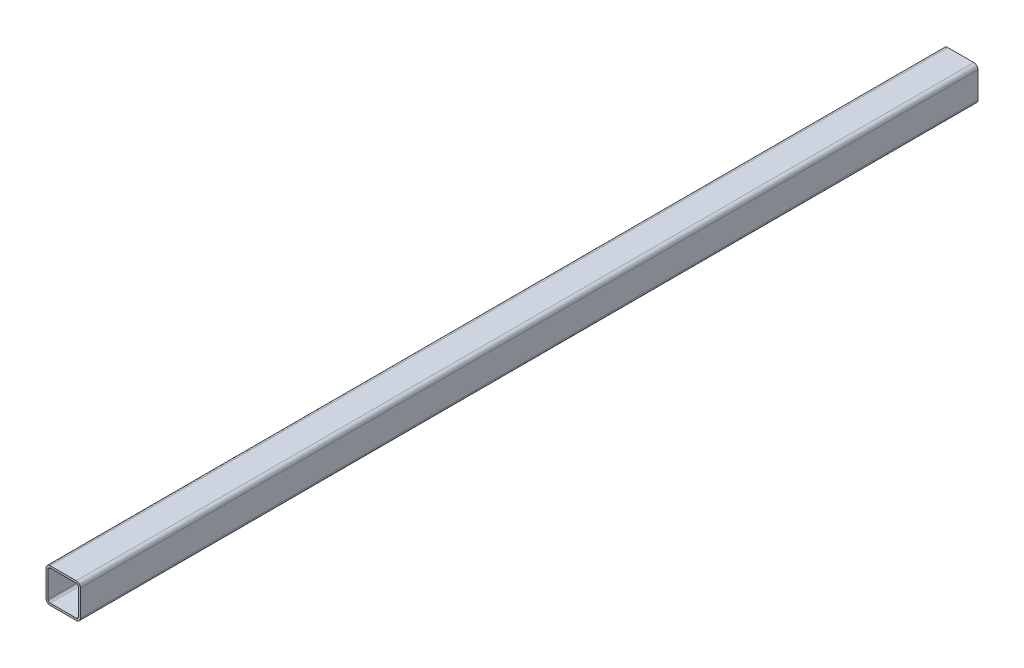
from build123d import *

# Parameters (mm, degrees)
GB_6728_1986_050_X_50_X_3_1_DEPTH = 1305


with BuildPart() as part:
    # Sketch1 → Gb／6728-1986方形空心型钢 050 X 50 X 3(1) (new body)
    with BuildSketch(Plane.YX.offset(-652.5)):
        with BuildLine():
            Line((-19, -25), (19, -25))
            ThreePointArc((19, -25), (23.242640687, -23.242640687), (25, -19))
            Line((25, -19), (25, 19))
            ThreePointArc((25, 19), (23.242640687, 23.242640687), (19, 25))
            Line((19, 25), (-19, 25))
            ThreePointArc((-19, 25), (-23.242640687, 23.242640687), (-25, 19))
            Line((-25, 19), (-25, -19))
            ThreePointArc((-25, -19), (-23.242640687, -23.242640687), (-19, -25))
        make_face()
        with BuildLine():
            Line((-19, -22), (19, -22))
            ThreePointArc((19, -22), (21.121320344, -21.121320344), (22, -19))
            Line((22, -19), (22, 19))
            ThreePointArc((22, 19), (21.121320344, 21.121320344), (19, 22))
            Line((19, 22), (-19, 22))
            ThreePointArc((-19, 22), (-21.121320344, 21.121320344), (-22, 19))
            Line((-22, 19), (-22, -19))
            ThreePointArc((-22, -19), (-21.121320344, -21.121320344), (-19, -22))
        make_face(mode=Mode.SUBTRACT)
    extrude(amount=GB_6728_1986_050_X_50_X_3_1_DEPTH)


solid = part.part
